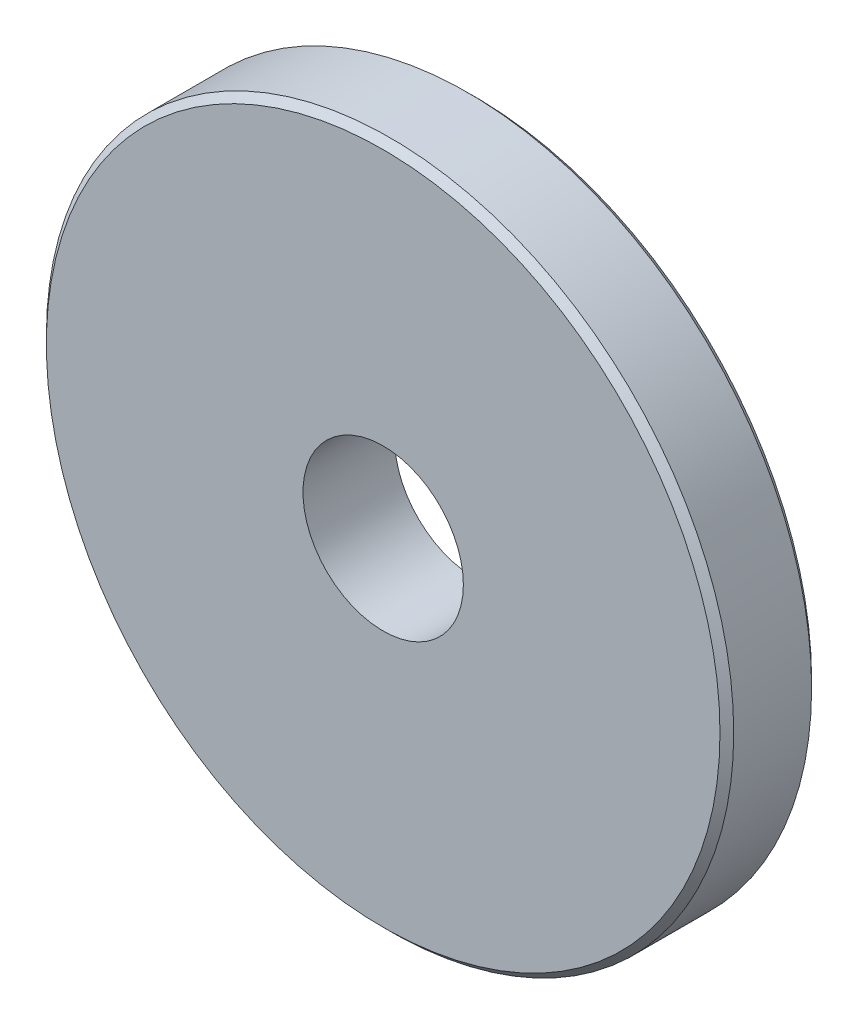
from build123d import *

# Parameters (mm, degrees)
SKETCH1_R           = 15
SKETCH1_R_2         = 3.5
BOSS_EXTRUDE1_DEPTH = 4
CHAMFER1_SIZE       = 0.3


with BuildPart() as part:
    # Sketch1 → Boss-Extrude1 (new body)
    with BuildSketch(Plane.XY):
        Circle(SKETCH1_R)
        Circle(SKETCH1_R_2, mode=Mode.SUBTRACT)
    extrude(amount=BOSS_EXTRUDE1_DEPTH)

    # Chamfer1
    chamfer1_edges = [part.edges().sort_by_distance(p)[0] for p in [
        (-15, 0, 0),
        (-15, 0, 4),
    ]]
    chamfer(chamfer1_edges, length=CHAMFER1_SIZE)


solid = part.part
